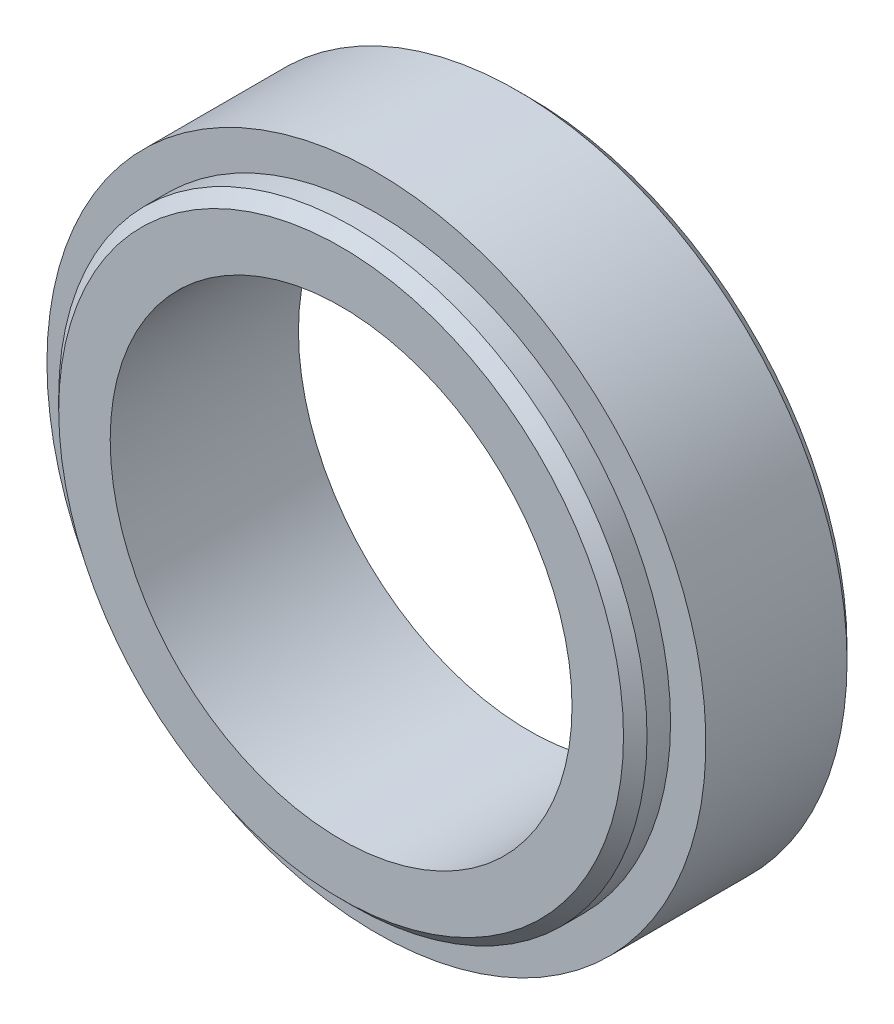
SolidWorks part; units mm, degrees
ref_plane "Front Plane" through (0, 0, 0) normal (0, 0, 1) x (1, 0, 0)
ref_plane "Top Plane" through (0, 0, 0) normal (0, 1, 0) x (1, 0, 0)
ref_plane "Right Plane" through (0, 0, 0) normal (1, 0, 0) x (0, 0, -1)
sketch "Sketch1" plane through (0, 0, 0) normal (0, 0, 1) x (1, 0, 0)
  circle A0 centre (0, 0) radius 28
extrude "Boss-Extrude1" add sketch "Sketch1" along normal blind 13
sketch "Sketch2" plane through (0, 0, 13) normal (0, 0, 1) x (1, 0, 0)
  circle A0 centre (0, 0) radius 25
extrude "Boss-Extrude2" add sketch "Sketch2" along normal blind 3
chamfer "Chamfer1" distance 1 distance2 1 2 edges at (28, 0, 0) (25, 0, 16)
sketch "Sketch3" plane through (0, 0, 16) normal (0, 0, 1) x (1, 0, 0)
  circle A0 centre (0, 0) radius 19.63
hole_wizard "G1-1/4 Tapped Hole1" positions "3DSketch1" profile "Sketch4" tap size "G1-1/4" standard "Gb"
sketch3d "3DSketch1"
  line L0 (0, 0, 15) -> (0, 0, 16) construction
  point P0 (0, 0, 0)
  point P3 (0, 0, 0)
  point P6 (0, 0, 16)
sketch "Sketch4" plane through (0, 0, 16) normal (1, 0, 0) x (0, -1, 0)
  line L0 (0, 0) -> (0, 102.5389)
  line L1 (0, 102.5389) -> (19.625, 90.747)
  line L2 (19.625, 90.747) -> (19.625, 0)
  line L5 (19.625, 0) -> (0, 0)
  line L10 (0, 102.5389) -> (-19.625, 90.747) construction
  line L11 (0, -6.35) -> (0, 107.95) construction
  dimension "螺纹孔钻头直径" = 39.25
  dimension "螺纹孔钻头深度" = 90.747
  dimension "导头角度" = 118
cosmetic thread "Hole Thread1" parameters "D1"=16, "D2"=41.91
cosmetic thread "Hole Thread2" parameters "D1"=16, "D2"=41.91
cosmetic thread "Hole Thread3" parameters "D1"=16, "D2"=41.91
sketch "Sketch5" plane through (0, 0, 16) normal (0, 0, 1) x (1, 0, 0)
